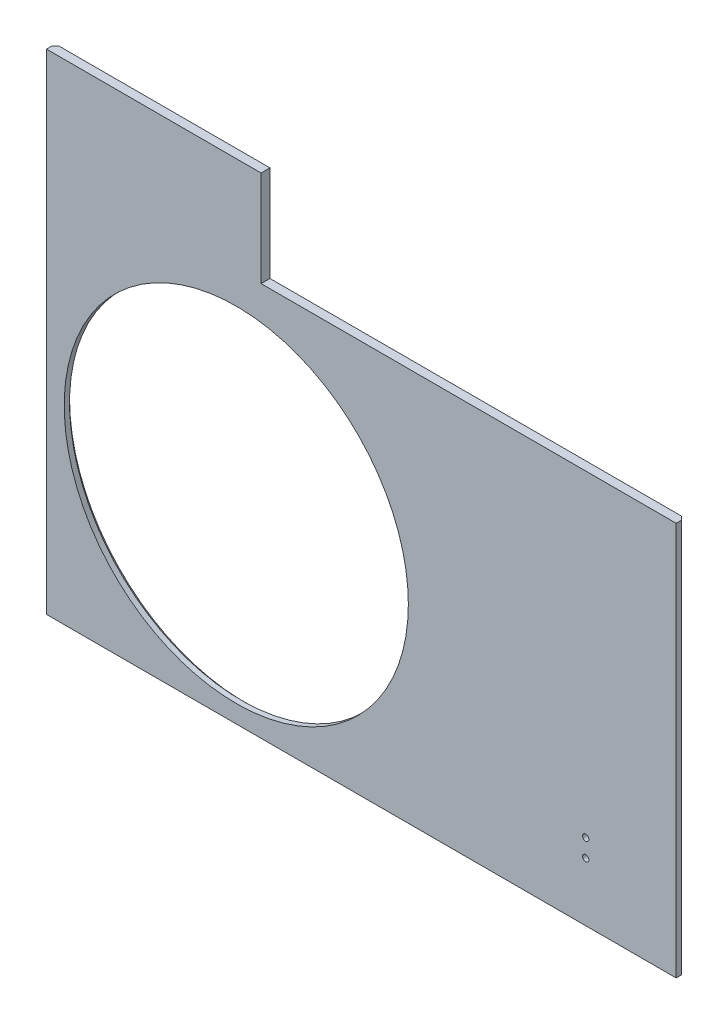
from build123d import *

# Parameters (mm, degrees)
SKETCH1_R            = 485
BOSS_EXTRUDE1_DEPTH  = 25
CHAMFER1_SIZE        = 10
M20_THREADED_HOLE1_D = 17.5


with BuildPart() as part:
    # Sketch1 → Boss-Extrude1 (new body)
    with BuildSketch(Plane.XY):
        Polygon((0, 0), (1775, 0), (1775, 1110), (605, 1110), (605, 1380), (0, 1380), align=None)
        with Locations((535, 535)):
            Circle(SKETCH1_R, mode=Mode.SUBTRACT)
    extrude(amount=BOSS_EXTRUDE1_DEPTH)

    # Chamfer1
    chamfer1_edges = [part.edges().sort_by_distance(p)[0] for p in [
        (50, 535, 0),
        (1775, 555, 0),
        (887.5, 0, 0),
        (0, 690, 0),
    ]]
    chamfer(chamfer1_edges, length=CHAMFER1_SIZE)

    # M20 Threaded hole1 (through all)
    with Locations(Plane(origin=(1520, 215, 0), x_dir=(-1, 0, 0), z_dir=(0, 0, -1))):
        with Locations((0, 0), (0, -50)):
            Hole(M20_THREADED_HOLE1_D / 2)


solid = part.part
